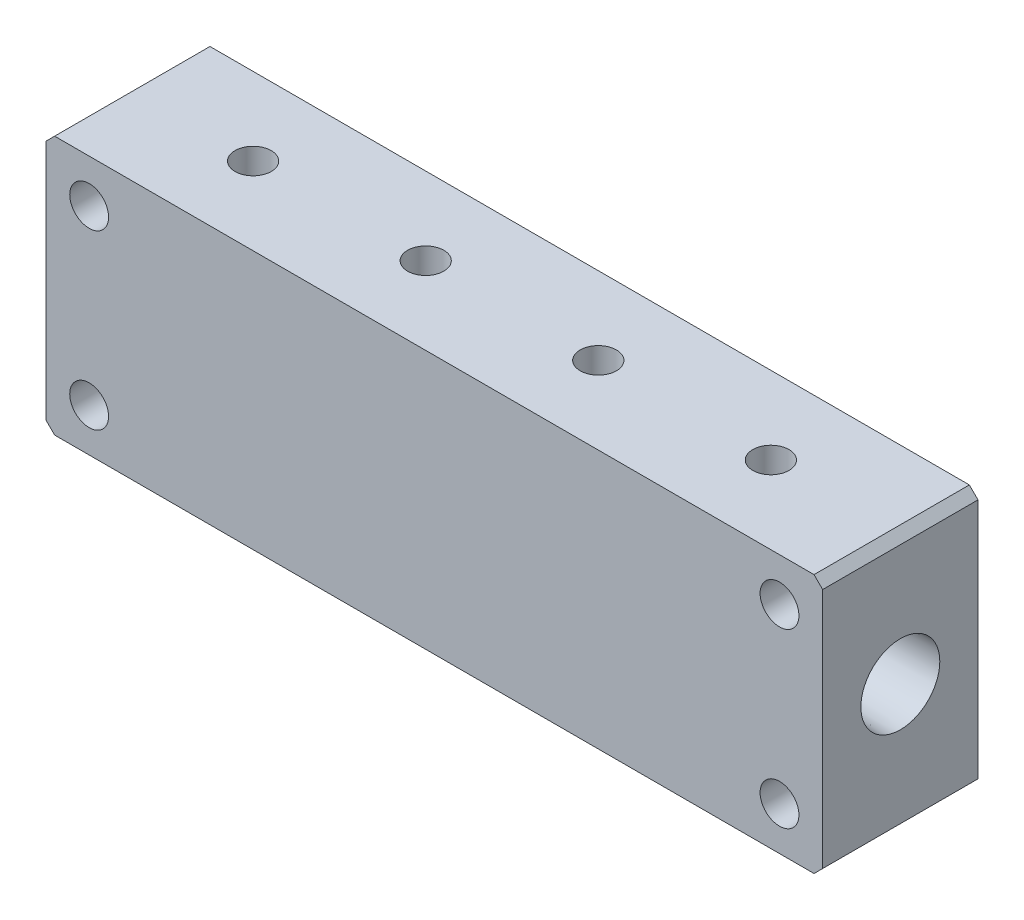
from build123d import *

# Parameters (mm, degrees)
SKETCH_1_W                = 90
SKETCH_1_H                = 18
EXTRUDE_1_DEPTH           = 15
HOLE_WIZARD_M5_1_D        = 4.2
HOLE_WIZARD_1_D           = 4.5
HOLE_WIZARD_1_CBORE_D     = 8
HOLE_WIZARD_1_CBORE_DEPTH = 4.6
CHAMFER_1_SIZE            = 1


with BuildPart() as part:
    # 草图1 → 凸台-拉伸1 (new, symmetric)
    with BuildSketch(Plane(origin=(0, 0, 0), x_dir=(1, 0, 0), z_dir=(0, 1, 0))):
        Rectangle(SKETCH_1_W, SKETCH_1_H)
    extrude(amount=EXTRUDE_1_DEPTH, both=True)

    # 草图4 → 1/8 Rc 螺纹孔2 (revolve, cut)
    with BuildSketch(Plane(origin=(45, 0, 0), x_dir=(0, 0, -1), z_dir=(0, 1, 0))):
        Polygon((0, 0), (0, 82.373399445), (3.95, 80), (3.95, 7.4), (4.342497004, 7.4), (4.5735, 0), align=None)
    revolve(axis=Axis((51.35, 0, 0), (-1, 0, 0)), mode=Mode.SUBTRACT)

    # M5 螺纹孔1 (through all)
    with Locations(Plane(origin=(0, 15, 0), x_dir=(1, 0, 0), z_dir=(0, 1, 0))):
        with Locations((30, 0), (10, 0), (-10, 0), (-30, 0)):
            Hole(HOLE_WIZARD_M5_1_D / 2)

    # 打孔尺寸(%根据)内六角圆柱头螺钉的类型1 (through all)
    with Locations(Plane(origin=(0, 0, -9), x_dir=(1, 0, 0), z_dir=(0, 0, -1))):
        with Locations((-40, -10), (-40, 10), (40, 10), (40, -10)):
            CounterBoreHole(HOLE_WIZARD_1_D / 2, HOLE_WIZARD_1_CBORE_D / 2, HOLE_WIZARD_1_CBORE_DEPTH)

    # 倒角1
    chamfer_1_edges = [part.edges().sort_by_distance(p)[0] for p in [
        (-45, 15, 0),
        (45, 15, 0),
        (-45, -15, 0),
        (45, -15, 0),
    ]]
    chamfer(chamfer_1_edges, length=CHAMFER_1_SIZE)


solid = part.part
